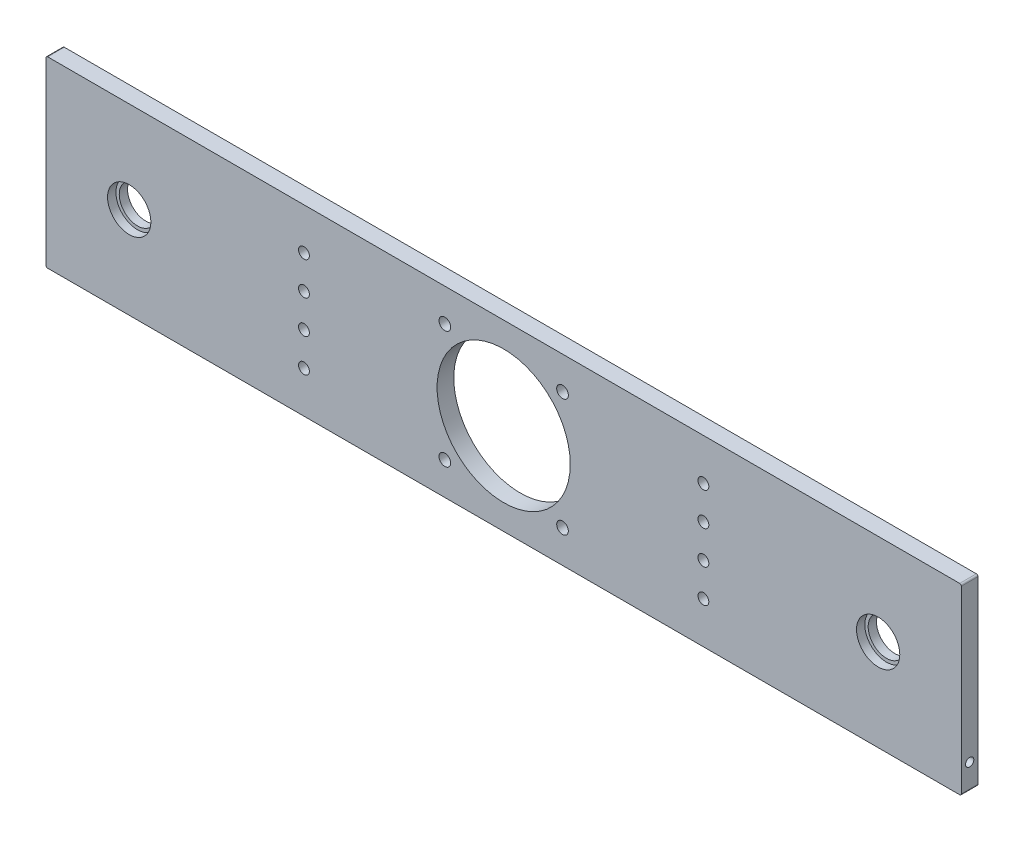
SolidWorks part; units mm, degrees
material "6061-T6 "
ref_plane "Front Plane" through (0, 0, 0) normal (0, 0, 1) x (1, 0, 0)
ref_plane "Top Plane" through (0, 0, 0) normal (0, 1, 0) x (1, 0, 0)
ref_plane "Right Plane" through (0, 0, 0) normal (1, 0, 0) x (0, 0, -1)
sketch "Sketch1" plane through (0, 0, 0) normal (0, 0, 1) x (1, 0, 0)
  line L1 (275, -55) -> (-275, -55)
  line L2 (275, -55) -> (275, 55)
  line L3 (275, 55) -> (-275, 55)
  line L4 (-275, -55) -> (-275, 55)
  line L5 (275, -55) -> (-275, 55) construction
  line L6 (275, 55) -> (-275, -55) construction
  point P0 (0, 0)
  dimension "D1" = 110
  dimension "D2" = 550
extrude "Boss-Extrude1" add sketch "Sketch1" along normal blind 10
sketch "Sketch3" plane through (0, 0, 10) normal (0, 0, 1) x (1, 0, 0)
  line L0 (0, 55) -> (0, -55) construction
  line L1 (275, 55) -> (-275, 55) construction
  line L2 (-275, -55) -> (275, -55) construction
  circle A0 centre (225, 0) radius 13
  circle A1 centre (-225, 0) radius 13
  dimension "D1" = 26
  dimension "D2" = 225
extrude "Cut-Extrude2" cut sketch "Sketch3" against normal blind 5
sketch "Sketch4" plane through (0, 0, 5) normal (0, 0, 1) x (1, 0, 0)
  line L0 (0, 55) -> (0, -55) construction
  line L1 (275, 55) -> (-275, 55) construction
  line L2 (-275, -55) -> (275, -55) construction
  circle A0 centre (225, 0) radius 11
  circle A1 centre (-225, 0) radius 11
  dimension "D1" = 22
extrude "Cut-Extrude3" cut sketch "Sketch4" against normal through all
sketch "Sketch5" plane through (0, 0, 10) normal (0, 0, 1) x (1, 0, 0)
  circle A0 centre (0, 0) radius 40
  dimension "D1" = 80
extrude "Cut-Extrude4" cut sketch "Sketch5" against normal through all
sketch "Sketch6" plane through (0, 0, 10) normal (0, 0, 1) x (1, 0, 0)
  line L0 (-35.3553, 35.3553) -> (35.3553, -35.3553) construction
  line L1 (-35.3553, -35.3553) -> (35.3553, 35.3553) construction
  line L2 (0, 0) -> (50, 0) construction
  circle A0 centre (0, 0) radius 50 construction
  circle A1 centre (-35.3553, 35.3553) radius 3.5
  circle A2 centre (35.3553, 35.3553) radius 3.5
  circle A3 centre (35.3553, -35.3553) radius 3.5
  circle A4 centre (-35.3553, -35.3553) radius 3.5
  dimension "D1" = 100
  dimension "D4" = 7
  dimension "D2" = 45
  dimension "D3" = 90
extrude "Cut-Extrude5" cut sketch "Sketch6" against normal through all
sketch "Sketch7" plane through (0, 0, 10) normal (0, 0, 1) x (1, 0, 0)
  line L0 (0, 55) -> (0, -55) construction
  line L1 (275, 55) -> (-275, 55) construction
  line L2 (-275, -55) -> (275, -55) construction
  line L3 (-275, 0) -> (275, 0) construction
  line L4 (-275, 55) -> (-275, -55) construction
  line L5 (275, -55) -> (275, 55) construction
  circle A2 centre (-120, -10) radius 3.25
  circle A3 centre (120, -10) radius 3.25
  circle A4 centre (120, 10) radius 3.25
  circle A5 centre (-120, 10) radius 3.25
  circle A6 centre (-120, -30) radius 3.25
  circle A7 centre (-120, 30) radius 3.25
  circle A8 centre (120, 30) radius 3.25
  circle A9 centre (120, -30) radius 3.25
  dimension "D2" = 20
  dimension "D1" = 240
  dimension "D3" = 6.5
  dimension "D4" = 60
  dimension "D5" = 60
extrude "Cut-Extrude6" cut sketch "Sketch7" against normal through all
fillet "Fillet1" radius 1 4 edges at (-275, -55, 5) (-275, 55, 5) (275, -55, 5) (275, 55, 5)
hole_wizard "M6 Tapped Hole1" positions "Sketch8" profile "Sketch9" tap size "M6" standard "GB"
sketch "Sketch8" plane through (-275, 0, 0) normal (-1, 0, 0) x (0, 0, 1)
  line L0 (10, 54) -> (0, 54) construction
  line L1 (10, -55) -> (0, -55) construction
  point P0 (5, -40)
  point P7 (5, 54)
  dimension "D1" = 15
sketch "Sketch9" plane through (-275, -40, 5) normal (0, 1, 0) x (0, 0, 1)
  line L0 (0, 0) -> (0, 19.5022)
  line L1 (0, 19.5022) -> (2.5, 18)
  line L2 (2.5, 18) -> (2.5, 0)
  line L5 (2.5, 0) -> (0, 0)
  line L10 (0, 19.5022) -> (-2.5, 18) construction
  line L11 (0, -6.35) -> (0, 107.95) construction
  dimension "螺纹孔钻头直径" = 5
  dimension "螺纹孔钻头深度" = 18
  dimension "导头角度" = 118
cosmetic thread "Hole thread1" parameters "D1"=15, "D2"=6
mirror "Mirror1" about plane through (0, 0, 0) normal (1, 0, 0) of "M6 Tapped Hole1"
